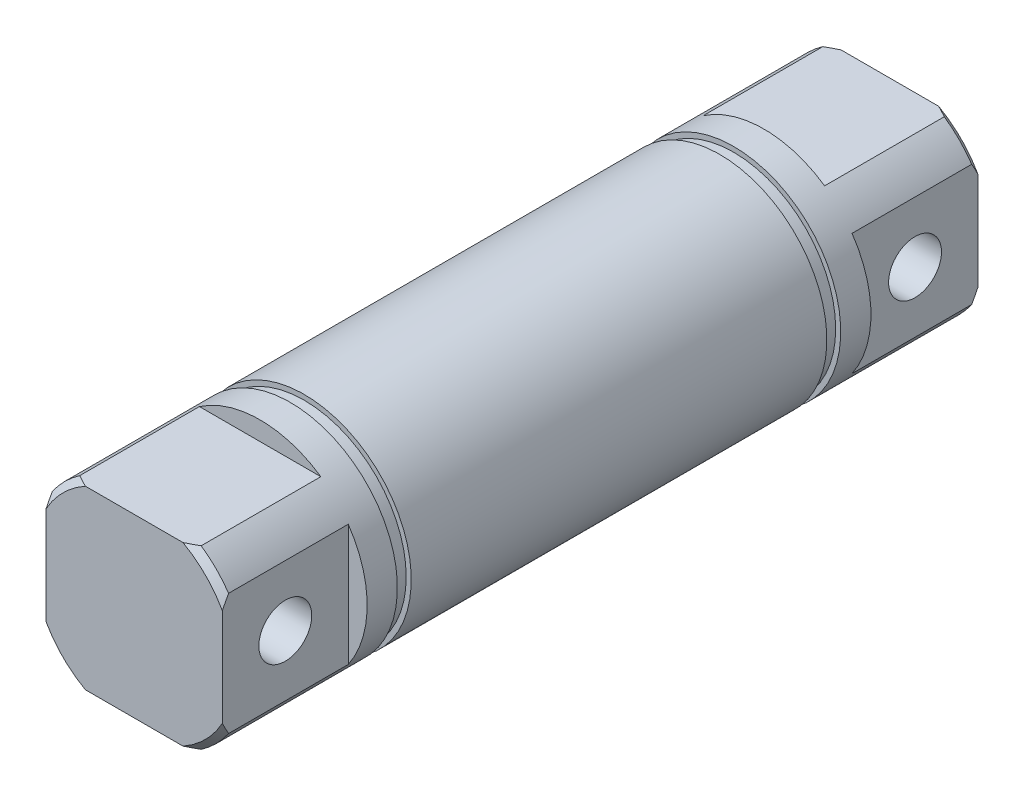
SolidWorks part; units mm, degrees
ref_plane "前视基准面" through (0, 0, 0) normal (0, 0, 1) x (1, 0, 0)
ref_plane "上视基准面" through (0, 0, 0) normal (0, 1, 0) x (1, 0, 0)
ref_plane "右视基准面" through (0, 0, 0) normal (1, 0, 0) x (0, 0, -1)
sketch "草图1" plane through (0, 0, 0) normal (0, 0, 1) x (1, 0, 0)
  circle A0 centre (0, 0) radius 8.5
  dimension "D1" = 17
extrude "凸台-拉伸1" add sketch "草图1" along normal mid plane 60
sketch "草图4" plane through (0, 0, 30) normal (0, 0, 1) x (1, 0, 0)
  line L1 (-7, 7) -> (7, 7)
  line L2 (-7, 7) -> (-7, -7)
  line L3 (-7, -7) -> (7, -7)
  line L4 (7, 7) -> (7, -7)
  line L5 (-7, 7) -> (7, -7) construction
  line L6 (-7, -7) -> (7, 7) construction
  point P0 (0, 0)
  dimension "D1" = 14
  dimension "D2" = 14
extrude "切除-拉伸1" cut sketch "草图4" against normal blind 10 flip side to cut
hole_wizard "M5 螺纹孔1" positions "草图6" profile "草图5" tap size "M5" standard "ISO" end condition up to next
sketch "草图6" plane through (7, 0, 0) normal (1, 0, 0) x (0, 0, -1)
  line L0 (-30, -4.8218) -> (-30, 4.8218) construction
  point P0 (-25, 0)
  dimension "D1" = 5
sketch "草图5" plane through (7, 0, 25) normal (0, 1, 0) x (0, 0, -1)
  line L0 (0, 0) -> (0, 14.001)
  line L1 (0, 14.001) -> (2.1, 14.001)
  line L2 (2.1, 14.001) -> (2.1, 0)
  line L5 (2.1, 0) -> (0, 0)
  line L11 (0, -6.35) -> (0, 107.95) construction
  dimension "通孔螺纹孔钻头直径" = 4.2
  dimension "通孔螺纹孔钻头深度" = 14.001
cosmetic thread "孔螺蚊线1" parameters "D2"=5
mirror "镜向1" about plane through (0, 0, 0) normal (0, 0, 1) of "M5 螺纹孔1", "切除-拉伸1"
chamfer "倒角1" distance 0.5 angle 45 12 edges at (0, 7, 30) (-7, 0, 30) (0, -7, 30) (7, 0, 30) (6.0104, -6.0104, 30) (-6.0104, -6.0104, 30) (-6.0104, 6.0104, 30) (6.0104, 6.0104, 30) (6.0104, -6.0104, -30) (6.0104, 6.0104, -30) (-6.0104, 6.0104, -30) (-6.0104, -6.0104, -30)
sketch "草图7" plane through (0, 0, 0) normal (0, 1, 0) x (1, 0, 0)
  line L0 (0, 14.7653) -> (0, 0) construction
  line L1 (0, 0) -> (26.0827, 0) construction
  line L2 (8.5, -20) -> (8.5, 20) construction
  line L3 (8.5, 17.6) -> (8.1, 17.6)
  line L4 (8.5, 17.6) -> (8.5, 16.5)
  line L5 (8.5, 16.5) -> (8.1, 16.5)
  line L6 (8.1, 17.6) -> (8.1, 16.5)
  dimension "D1" = 1.1
  dimension "D2" = 16.5
  dimension "D3" = 8.1
revolve "切除-旋转1" cut sketch "草图7" angle 360 about L0
mirror "镜向2" about plane through (0, 0, 0) normal (0, 0, 1) of "切除-旋转1"
